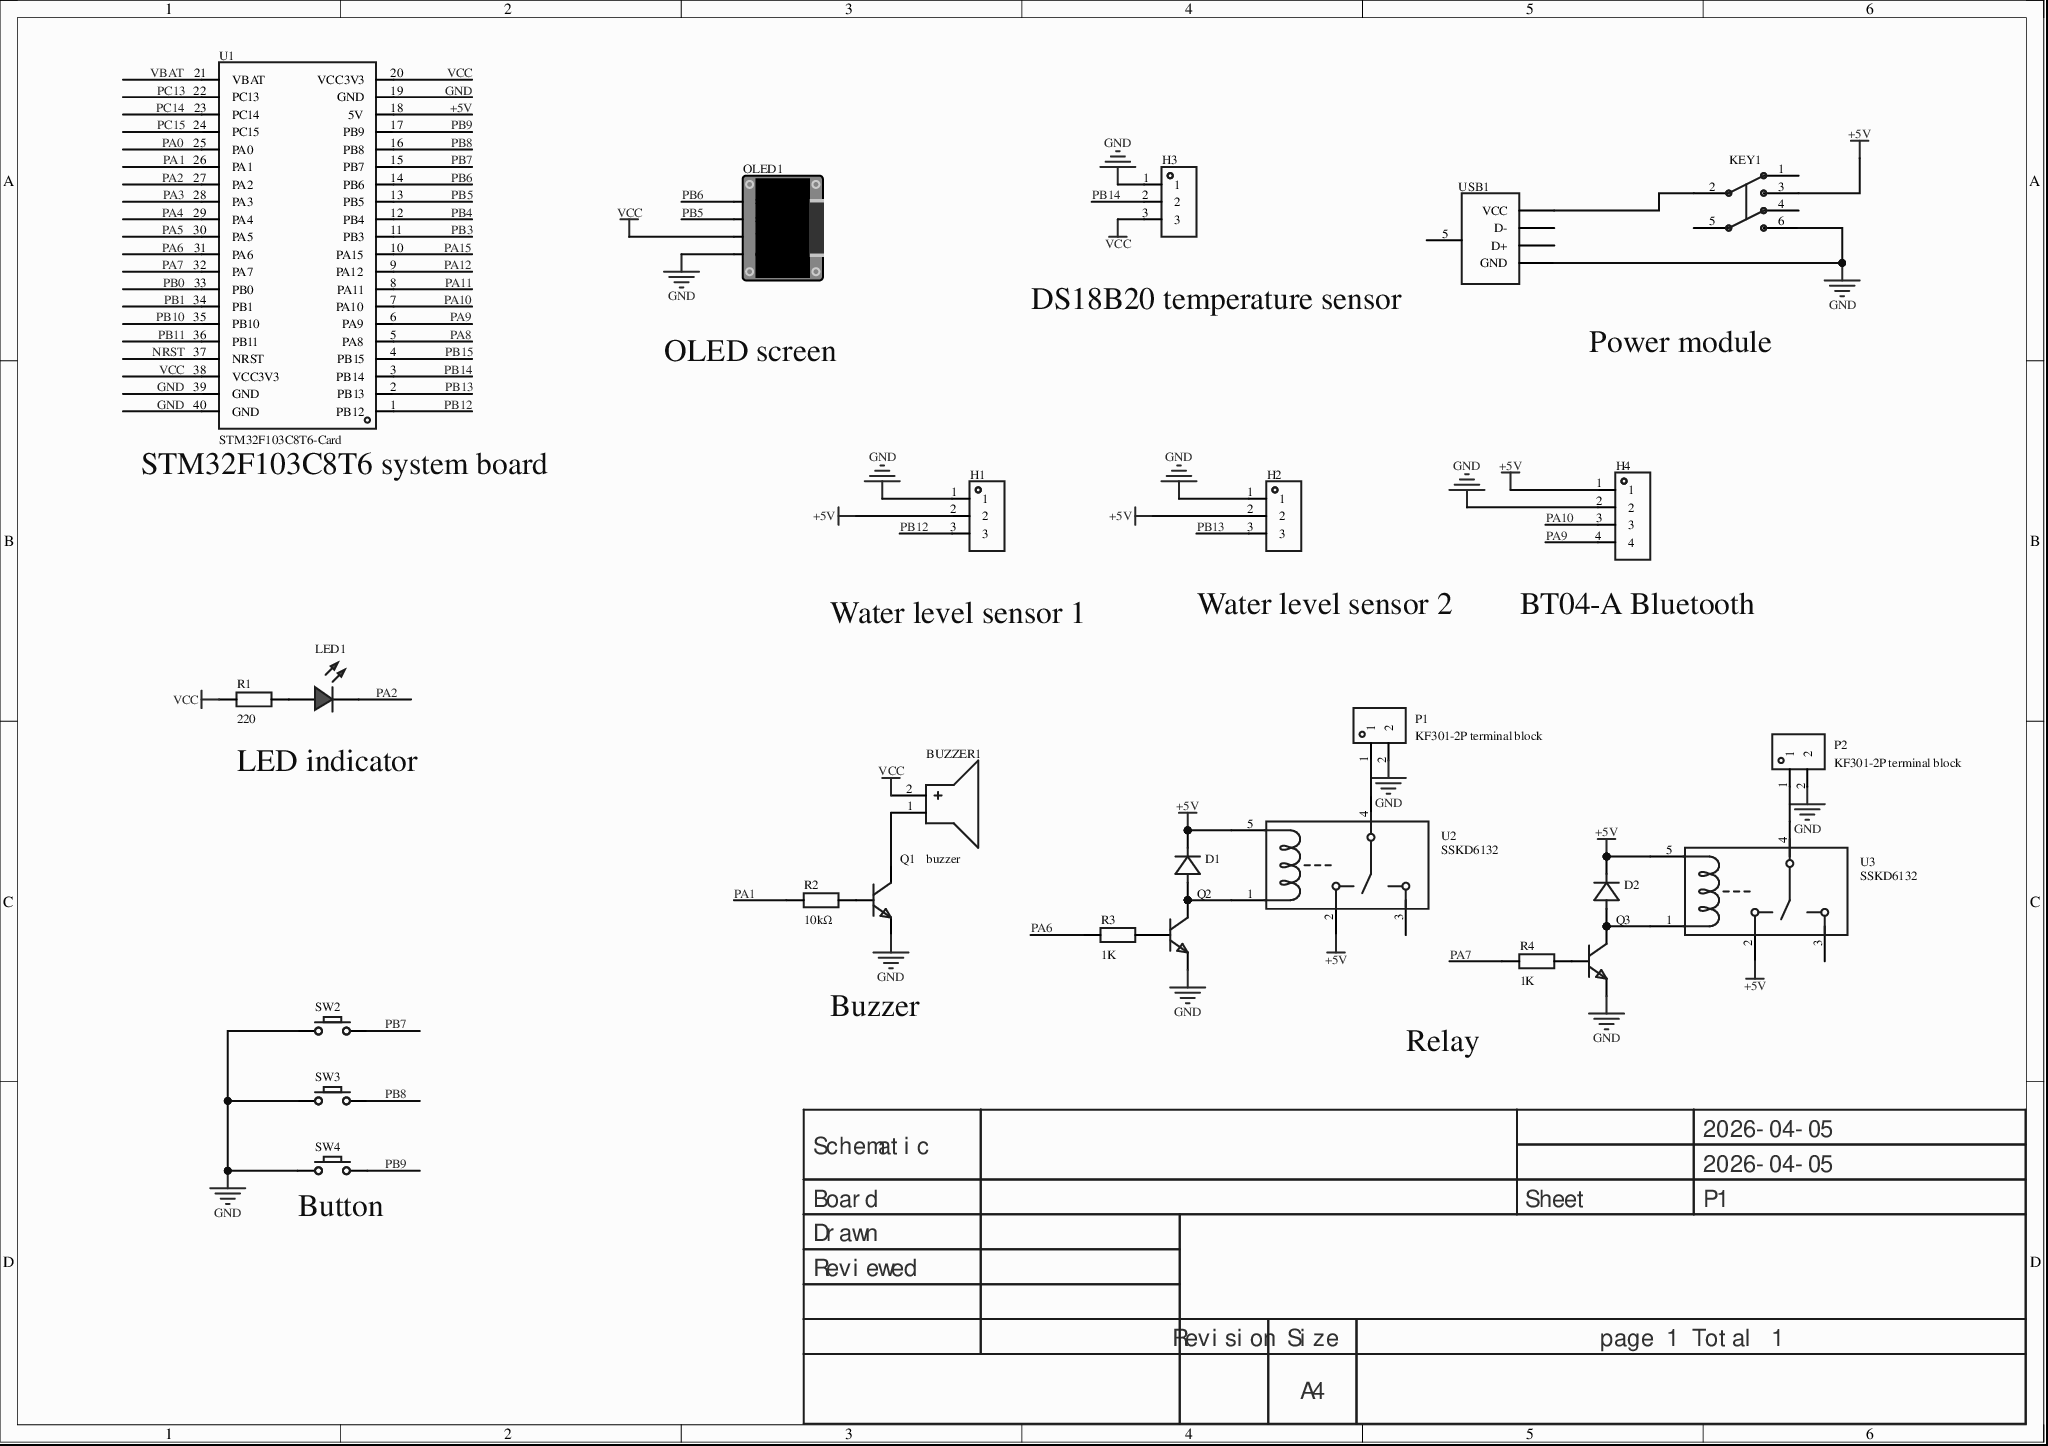
[diagram p0: MISC89014-3.schdoc]
# Altium project MISC89014-2.PrjPcb
1 sheet, 26 parts. Net scope: global (net labels, ports and power ports of the same name join across sheets).
Board file: MISC89014.pcbdoc

## Sheet MISC89014-3.schdoc
size 297 x 209 mm; Version: V1.0; @Project Name: MISC89014; @Page Count: 1; @Update Date: 2026-04-05; @Create Date: 2026-04-05; @Schematic Name: MISC89014; @Page No: 1; @Create Time: 18:58:15; @Update Time: 22:44:58; @Board Name: MISC89014

### Parts
BUZZER1  buzzer  [BUZ-TH_BD12.0-P6.00-D0.9-RD]
D1  (no value)  [SMA_1N4007]
D2  (no value)  [SMA_1N4007]
H1  (no value)  [HDR-TH_3P-P2.54-V-F]
H2  (no value)  [HDR-TH_3P-P2.54-V-F]
H3  (no value)  [HDR-TH_3P-P2.54-V-F]
H4  (no value)  [HDR-TH_4P-P2.54-V-F]
KEY1  Non-self-locking switch 8.5×8.5 silent  [SW-TH_6P-L8.5-W8.5-P2.54]  (value not drawn)
LED1  (no value)  [LED_TH-3mm]
OLED1  (no value)  [0.96OLED_4P]
P1  KF301-2P terminal block  [CONN-TH_XY301V-A-5.0-2P]
P2  KF301-2P terminal block  [CONN-TH_XY301V-A-5.0-2P]
Q1  (no value)  [S8050_TO_92]
Q2  (no value)  [S8050_SOT-23]
Q3  (no value)  [S8050_SOT-23]
R1  220  [Res_1/8W]
R2  10kΩ  [Res_1/8W]
R3  1K  [R0603]
R4  1K  [R0603]
SW2  (no value)  [Key_TH_3.5x6x4.3]
SW3  (no value)  [Key_TH_3.5x6x4.3]
SW4  (no value)  [Key_TH_3.5x6x4.3]
U1  STM32F103C8T6-Card  [CONN-TH_L53.3-W22.9_STM32F103C8T6-CARD]
U2  SSKD6132  [RELAY-TH_G2R-1]
U3  SSKD6132  [RELAY-TH_G2R-1]
USB1  (no value)  [USB_ Type-B]

### Nets
+5V: D1.1(K) D2.1(K) H1.2 H2.2 H4.1 KEY1.3 U1.18(5V) U2.2 U2.5 U3.2 U3.5
GND: H1.1 H2.1 H3.1 H4.2 KEY1.6 OLED1.1(GND) P1.2 P2.2 Q1.1(E) Q2.2 Q3.2 SW2.A SW3.A SW4.A U1.19(GND) U1.39(GND) U1.40(GND) USB1.4(GND)
VCC: BUZZER1.2(+) H3.3 OLED1.2(VCC) R1.1 U1.20(VCC3V3) U1.38(VCC3V3)
NRST: U1.37(NRST)
PA0: U1.25(PA0)
PA1: R2.1 U1.26(PA1)
PA2: LED1.2(A) U1.27(PA2)
PA3: U1.28(PA3)
PA4: U1.29(PA4)
PA5: U1.30(PA5)
PA6: R3.1 U1.31(PA6)
PA7: R4.1 U1.32(PA7)
PA8: U1.5(PA8)
PA9: H4.4 U1.6(PA9)
PA10: H4.3 U1.7(PA10)
PA11: U1.8(PA11)
PA12: U1.9(PA12)
PA15: U1.10(PA15)
PB0: U1.33(PB0)
PB1: U1.34(PB1)
PB3: U1.11(PB3)
PB4: U1.12(PB4)
PB5: OLED1.3(SCL) U1.13(PB5)
PB6: OLED1.4(SDA) U1.14(PB6)
PB7: SW2.B U1.15(PB7)
PB8: SW3.B U1.16(PB8)
PB9: SW4.B U1.17(PB9)
PB10: U1.35(PB10)
PB11: U1.36(PB11)
PB12: H1.3 U1.1(PB12)
PB13: H2.3 U1.2(PB13)
PB14: H3.2 U1.3(PB14)
PB15: U1.4(PB15)
PC13: U1.22(PC13)
PC14: U1.23(PC14)
PC15: U1.24(PC15)
VBAT: U1.21(VBAT)
NetBUZZER1_1: BUZZER1.1(-) Q1.3(C)
NetD1_2: D1.2(A) Q2.3 U2.1
NetD2_2: D2.2(A) Q3.3 U3.1
NetKEY1_2: KEY1.2 USB1.1(VCC)
NetLED1_1: LED1.1(C) R1.2
NetP1_1: P1.1 U2.4
NetP2_1: P2.1 U3.4
NetQ1_2: Q1.2(B) R2.2
NetQ2_1: Q2.1 R3.2
NetQ3_1: Q3.1 R4.2

Not connected (* = marked no-connect by the designer): KEY1 1 4 5; U2 3; U3 3; USB1 2(D-)* 3(D+)* 5(SH1)

### Notes on the sheet
- (near USB1) DS18B20 temperature sensor
- OLED screen
- Power module
- (near U1) STM32F103C8T6 system board
- (near H1) Water level sensor 1
- (near H2) Water level sensor 2
- (near H4) BT04-A Bluetooth
- LED indicator
- Buzzer
- Relay
- (near SW4) Button
- 2026-04-05
- Schematic
- Board
- Sheet
- P1
- Drawn
- Reviewed
- Revision
- Size
- A4
- page 1 Total 1

### Library data of the parts
BUZZER1 = buzzer: AddInBom: yes; ModelId: af17e4151ed84fc2a628230bf23763630819f05c4eef4c71ace90d822a990e87; ModelTransform: 472.44,472.176,0,270,0,0,0,0,-196.85; Symbol: BUZZER; Device: buzzer; LCSC Part Name: buzzer; SupplierPart: C9900014030; ManufacturerPart: buzzer; Supplier Footprint: buzzer; JLCPCB Part Class: Extended Part; Supplier: LCSC; ConvertToPcb: yes; FootprintName: BUZ-TH_BD12.0-P6.00-D0.9-RD; ModelName: BUZ-TH_BD12.0-P6.00-D0.9-RD
D1 D2 = D_1N4007: AddInBom: yes; ModelId: 4f1e9ef2303f48b48aa8ce0cacf8d7b10819f05c4eef4c71ace90d822a990e87; ModelName: SMA_L4.4-W2.8-LS5.4-RD; ModelTransform: 204.7,102.4,82.7,0,0,0,0,0,0; Symbol: D_1N4007; Device: D_1N4007; ConvertToPcb: yes; FootprintName: SMA_1N4007; Supplier Footprint: SMA
H1 H2 = HDR-F_2.54_1x3P: Symbol: PM254V-11-03-H85; 3D Model: f3b3cc5aae9641bf9e56fc160cef875b; 3D Model Transform: 299.9994,100,0,0,0,0,0,0,-118.11; ConvertToPcb: yes; ModelName: HDR2.54-F-LI-1X3P; Device: HDR-F_2.54_1x3P; Supplier Part: C541850; Supplier Footprint: 插件; AddInBom: yes; FootprintName: HDR-TH_3P-P2.54-V-F
H3 = HDR-F_2.54_1x3P: Symbol: PM254V-11-03-H85; ConvertToPcb: yes; ModelId: f3b3cc5aae9641bf9e56fc160cef875b; ModelName: HDR2.54-F-LI-1X3P; ModelTransform: 299.9994,100,0,0,0,0,0,0,-118.11; Device: HDR-F_2.54_1x3P; AddInBom: yes; SupplierPart: C541850; Supplier Footprint: 插件; FootprintName: HDR-TH_3P-P2.54-V-F
H4 = HDR-F_2.54_1x4P: Symbol: 2.54-1*4P female; ConvertToPcb: yes; ModelId: d187812051054f85879fcaa51a310d8e0819f05c4eef4c71ace90d822a990e87; ModelTransform: 419.6842,98.464,0,0,0,0,0,0,-118.11; Device: HDR-F_2.54_1x4P; AddInBom: yes; SupplierPart: C2718488; Supplier Footprint: 插件; FootprintName: HDR-TH_4P-P2.54-V-F; ModelName: HDR-TH_4P-P2.54-V-F
KEY1 = 无自锁开关 8.5×8.5 无声: 6-pin, 8.5×8.5; Symbol: No self-locking switch 8.5×8.5 silent; AddInBom: yes; ModelId: 4c72b3966b92446eb355e1bd0fb4f8800819f05c4eef4c71ace90d822a990e87; ModelTransform: 342.519,334.645,0,180,0,0,0,0,-137.795; Device: Non-self-locking switch 8.5×8.5 silent; LCSC Part Name: 无自锁开关 8.5×8.5  无声; SupplierPart: C26228; ManufacturerPart: 无自锁开关 8.5×8.5 无声; Supplier Footprint: 插件; JLCPCB Part Class: Extended Part; Supplier: LCSC; ConvertToPcb: yes; FootprintName: SW-TH_6P-L8.5-W8.5-P2.54; ModelName: SW-TH_6P-L8.5-W8.5-P2.54
LED1 = LED_TH-R_3mm: ConvertToPcb: yes; ModelId: a497c992633541038a38947cdc58012f0819f05c4eef4c71ace90d822a990e87; ModelName: LED-TH-3mm_R; ModelTransform: 141.274,153.327,0,0,0,0,-5.984,0,-137.795; Symbol: LED_TH-R; Device: LED_TH-R_3mm; AddInBom: yes; FootprintName: LED_TH-3mm; Supplier Footprint: 插件
OLED1 = 0.96OLED模块_4P: Symbol: 0.96OLED module_4P; ConvertToPcb: yes; ModelId: 79c000fdb68d45a296c2e9bedf4f9055; ModelTransform: 1393.69792,1318.895,0,0,0,0,0,-560.079,-137.795; Device: 0.96OLED module_4P; AddInBom: yes; FootprintName: 0.96OLED_4P; Supplier Footprint: 插件; ModelName: 0.96OLED_4P
P1 P2 = KF301-2P接线端子: AddInBom: yes; ModelId: ef7ead88b0f2448d904975b26718870f; ModelTransform: 417.322,299.212,0,0,0,0,11.811,-7.835,-157.48; Symbol: KF301-2P terminal block; Device: KF301-2P terminal block; LCSC Part Name: KF301-2P接线端子; SupplierPart: C9900016950; ManufacturerPart: KF301-2P接线端子; Supplier Footprint: CK301-2P; Supplier: LCSC; ConvertToPcb: yes; FootprintName: CONN-TH_XY301V-A-5.0-2P; ModelName: CONN-TH_XY301V-A-5.0-2P
Q1 = S8050_TO_NPN: ConvertToPcb: yes; ModelId: aafe8e06f2154e7c93506efd0d6632dd; ModelName: TO-92-3_L4.9-W3.7-P1.27-L; ModelTransform: 180.78,141.44,417.3,0,0,0,0,0,-200; Symbol: S8050_TO_NPN; Device: S8050_TO_NPN; AddInBom: yes; Supplier Footprint: TO-92; FootprintName: S8050_TO_92
Q2 Q3 = S8050_SOT_NPN: Symbol: NPN; ConvertToPcb: yes; ModelId: c62791f0466c4ae2a892c056b845b0ca0819f05c4eef4c71ace90d822a990e87; ModelName: SOT-23-3P_L2.9-W1.3-H1.0-LS2.4-P0.95; ModelTransform: 98.6,114.12,41.29,180,0,0,0,0,-3; Device: S8050_SOT_NPN; AddInBom: yes; Supplier Footprint: SOT-23; FootprintName: S8050_SOT-23
R1 R2 = Res_AXIAL-1/8W: Symbol: Resistor; ConvertToPcb: yes; ModelId: b2b5ae7ae4c642178fe0039925c86a3f; ModelName: RES-TH_BD1.8-L3.2-P7.20-D0.4; ModelTransform: 282.86,66.88,253.09,0,0,0,0,0,-191; Device: Res_AXIAL-1/8W; AddInBom: yes; Supplier Footprint: 轴向引线; FootprintName: Res_1/8W
  R1: Value: 220
  R2: Value: 10kΩ
R3 R4 = Res_0603: Symbol: Resistor; ConvertToPcb: yes; ModelId: fc143cca1e79419f9cd78b61e9279f080819f05c4eef4c71ace90d822a990e87; ModelTransform: 31.8897,63.7794,0,90,0,0,0,0,0; Device: Res_0603; Value: 1K; AddInBom: yes; Supplier Footprint: 0603; FootprintName: R0603; ModelName: R0603
SW2-SW4 = Key_TH_3.5x6x4.3: ConvertToPcb: yes; ModelId: c3523f9014d949d7ba5445190a3178990819f05c4eef4c71ace90d822a990e87; ModelName: SW-TH_L6.0-W3.5-H5.0-P6.5; ModelTransform: 308.49,137.8,335.08,0,0,0,0,0,-129.92; Symbol: Key_TH_3.5x6x4.3; Device: Key_TH_3.5x6x4.3; AddInBom: yes; Supplier Footprint: 插件; FootprintName: Key_TH_3.5x6x4.3
U1 = STM32F103C8T6-Card: AddInBom: yes; Symbol: STM32F103C8T6-CARD; Device: STM32F103C8T6-Card; LCSC Part Name: STM32F103C8T6-Card; SupplierPart: C9900077949; ManufacturerPart: STM32F103C8T6-Card; Supplier Footprint: 插件; Supplier: LCSC; ConvertToPcb: yes; FootprintName: CONN-TH_L53.3-W22.9_STM32F103C8T6-CARD
U2 U3 = SSKD6132: AddInBom: yes; ModelId: fe99462dd15043c98af5adb0e5338dda0819f05c4eef4c71ace90d822a990e87; ModelTransform: 1141.73,511.81,0,0,0,0,26.417,-0.354,-157.48; Symbol: SSKD6132; Device: SSKD6132; LCSC Part Name: SSKD6132; SupplierPart: C9900012103; ManufacturerPart: SSKD6132; Supplier Footprint: RELAY-TH_G2R-1; JLCPCB Part Class: Extended Part; Supplier: LCSC; ConvertToPcb: yes; FootprintName: RELAY-TH_G2R-1; ModelName: RELAY-TH_G2R-1
USB1 = USB_ Type-B: ConvertToPcb: yes; ModelId: bbf32347d5be4dcea8001c0804ac390e0819f05c4eef4c71ace90d822a990e87; ModelName: USB-B_TH_BF90; ModelTransform: 547.99,637.8,543.15,0,0,0,0,0,-125.98; Symbol: USB_ Type-B; Device: USB_ Type-B; AddInBom: yes; Supplier Footprint: 插件; FootprintName: USB_ Type-B